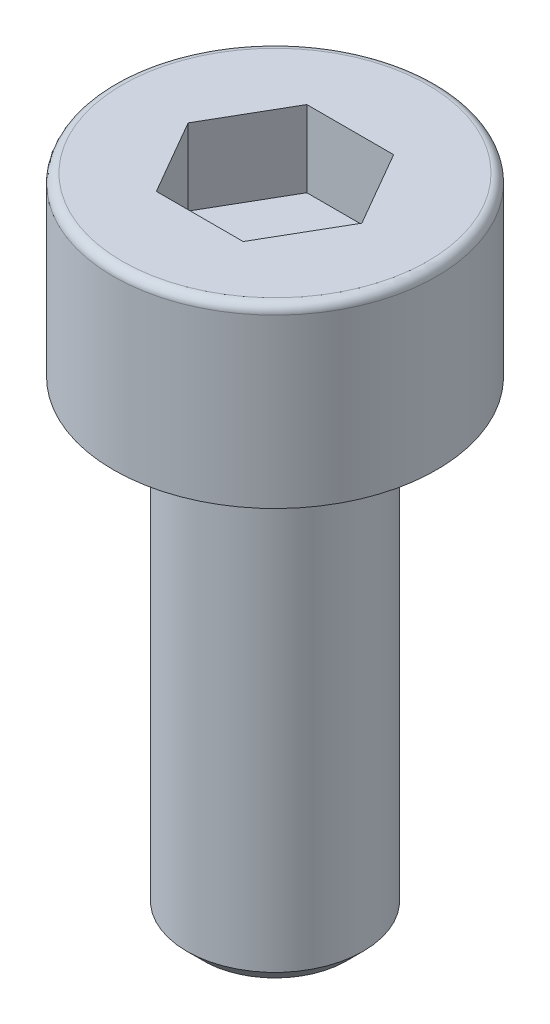
from build123d import *

# Parameters (mm, degrees)
SKETCH_1_R          = 2.75
EXTRUDE_1_DEPTH     = 3
CUT_EXTRUDE_1_DEPTH = 1.3
FILLET_1_R          = 0.15
SKETCH_5_R          = 1.5
EXTRUDE_2_DEPTH     = 8
CHAMFER_2_SIZE      = 0.28


with BuildPart() as part:
    # 草图1 → 凸台-拉伸1 (new body)
    with BuildSketch(Plane(origin=(0, 0, 0), x_dir=(1, 0, 0), z_dir=(0, 1, 0))):
        with Locations(Location((0, 0, 0), (0, 0, 270))):
            Circle(SKETCH_1_R)
    extrude(amount=EXTRUDE_1_DEPTH)

    # 草图2 → 切除-拉伸1 (cut)
    with BuildSketch(Plane(origin=(0, 3, 0), x_dir=(1, 0, 0), z_dir=(0, 1, 0))):
        Polygon((1.478016689, 0), (0.739008345, 1.28), (-0.739008345, 1.28), (-1.478016689, 0), (-0.739008345, -1.28), (0.739008345, -1.28), align=None)
    extrude(amount=-CUT_EXTRUDE_1_DEPTH, mode=Mode.SUBTRACT)

    # 圆角1
    fillet_1_edges = [part.edges().sort_by_distance(p)[0] for p in [
        (0, 3, -2.75),
    ]]
    fillet(fillet_1_edges, radius=FILLET_1_R)

    # 草图5 → 凸台-拉伸2 (add)
    with BuildSketch(Plane.XZ):
        with Locations(Location((0, 0, 0), (0, 0, 90))):
            Circle(SKETCH_5_R)
    extrude(amount=EXTRUDE_2_DEPTH)

    # 倒角2
    chamfer_2_edges = [part.edges().sort_by_distance(p)[0] for p in [
        (0, -8, -1.5),
    ]]
    chamfer(chamfer_2_edges, length=CHAMFER_2_SIZE)


solid = part.part
